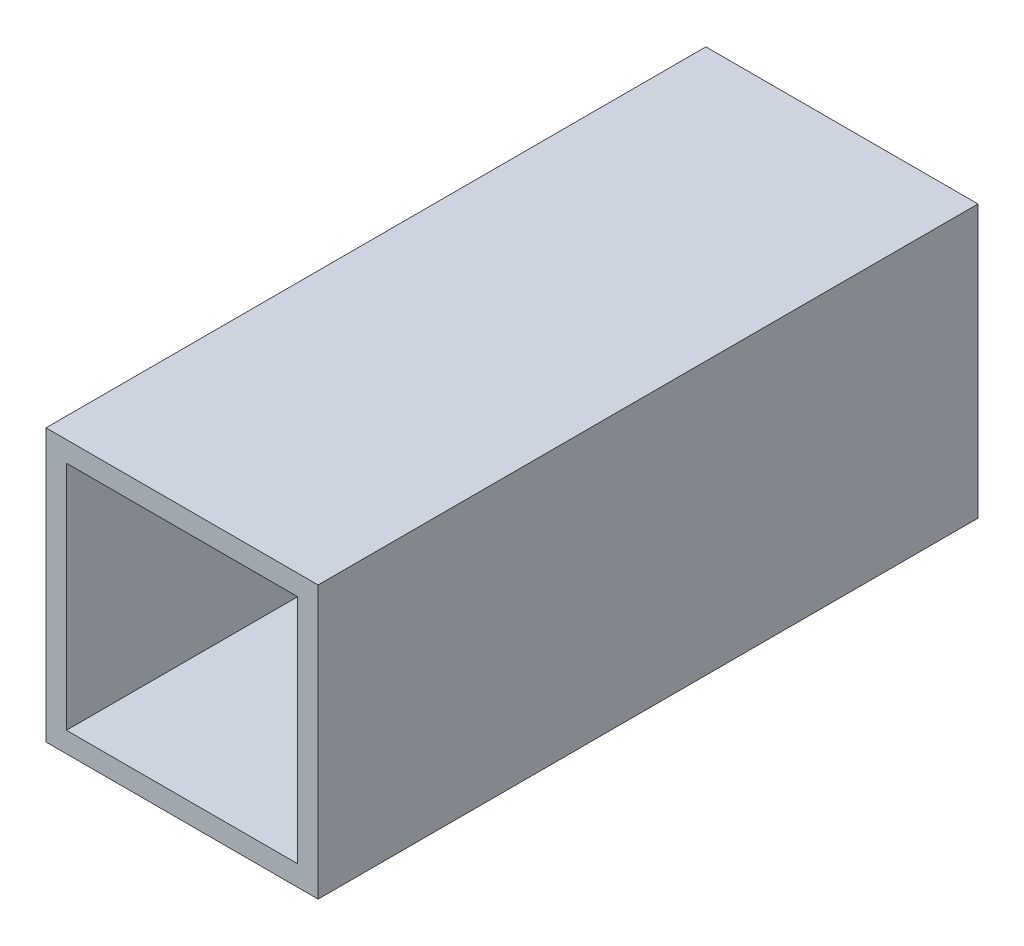
from build123d import *

# Parameters (mm, degrees)
SKETCH_1_W      = 40
SKETCH_1_H      = 40
SKETCH_1_W_2    = 34
SKETCH_1_H_2    = 34
EXTRUDE_1_DEPTH = 48.5


with BuildPart() as part:
    # 草图1 → 凸台-拉伸1 (new, symmetric)
    with BuildSketch(Plane.XY):
        Rectangle(SKETCH_1_W, SKETCH_1_H)
        Rectangle(SKETCH_1_W_2, SKETCH_1_H_2, mode=Mode.SUBTRACT)
    extrude(amount=EXTRUDE_1_DEPTH, both=True)


solid = part.part
